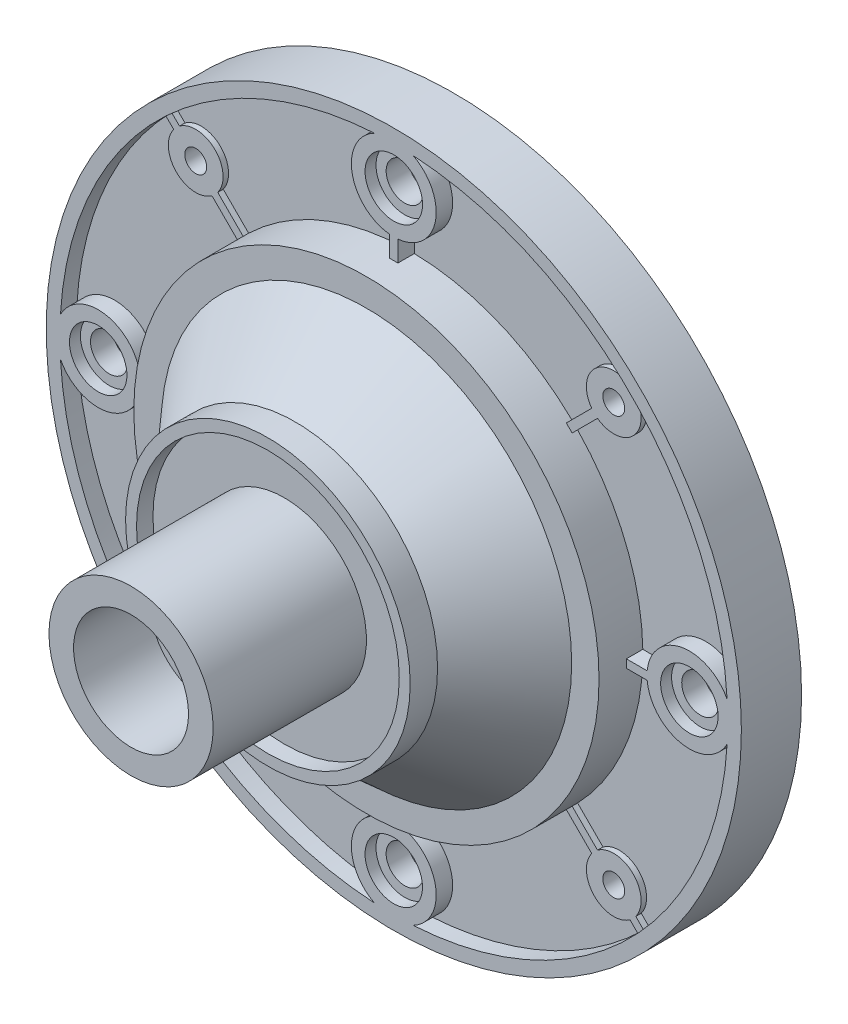
from build123d import *
from build123d.topology import SkipClean

# Parameters (mm, degrees)
SKETCH1_R           = 15
BOSS_EXTRUDE1_DEPTH = 30
SKETCH8_R           = 12
BOSS_EXTRUDE3_DEPTH = 20
SKETCH9_R           = 10.5
CUT_EXTRUDE3_DEPTH  = 14
SKETCH10_R          = 8.5
CUT_EXTRUDE4_DEPTH  = 42
SKETCH12_R          = 5.25
CUT_EXTRUDE5_DEPTH  = 2
SKETCH13_R          = 3.4
CUT_EXTRUDE6_DEPTH  = 16
CIRPATTERN1_COUNT   = 4
SKETCH15_R          = 5
CUT_EXTRUDE7_DEPTH  = 2
SKETCH16_R          = 2
CUT_EXTRUDE8_DEPTH  = 2
CIRPATTERN2_COUNT   = 4
CUT_EXTRUDE9_DEPTH  = 3
CUT_EXTRUDE10_DEPTH = 2
SKETCH19_R          = 2
CUT_EXTRUDE11_DEPTH = 36
SKETCH20_R          = 5.25
SKETCH20_R_2        = 3.4
BOSS_EXTRUDE4_DEPTH = 1
BOSS_EXTRUDE5_DEPTH = 12
BOSS_EXTRUDE6_REACH = 104.301
CIRPATTERN3_COUNT   = 8
BOSS_EXTRUDE9_START = -5
SKETCH25_W          = 1
SKETCH25_H          = 4.369199075
BOSS_EXTRUDE9_DEPTH = 3
CIRPATTERN4_COUNT   = 8


with BuildPart() as part:
    # Sketch1 → Boss-Extrude1 (new body)
    with BuildSketch(Plane.XY):
        Circle(SKETCH1_R)
    extrude(amount=BOSS_EXTRUDE1_DEPTH)

    # Sketch8 → Boss-Extrude3 (add)
    with BuildSketch(Plane(origin=(0, 0, 0), x_dir=(-1, 0, 0), z_dir=(0, 0, -1))):
        Circle(SKETCH8_R)
    extrude(amount=BOSS_EXTRUDE3_DEPTH)

    # Sketch9 → Cut-Extrude3 (cut)
    with BuildSketch(Plane.XY.offset(30)):
        Circle(SKETCH9_R)
    extrude(amount=-CUT_EXTRUDE3_DEPTH, mode=Mode.SUBTRACT)

    # Sketch10 → Cut-Extrude4 (cut)
    with BuildSketch(Plane.XY.offset(16)):
        Circle(SKETCH10_R)
    extrude(amount=-CUT_EXTRUDE4_DEPTH, mode=Mode.SUBTRACT)

    # Sketch11 → Revolve1 (revolve)
    with BuildSketch(Plane(origin=(0, 0, 0), x_dir=(0, 0, -1), z_dir=(1, 0, 0)), mode=Mode.PRIVATE) as revolve1_sk:
        Polygon((0, 12), (0, 23.329760776), (13.757661732, 35.5), (26, 35.5), (26, 37.5), (15, 37.5), (15, 40.5), (23, 40.5), (23, 61.5), (29, 61.5), (29, 63.5), (18, 63.5), (18, 42.5), (13, 42.5), (13, 37.5), (0, 26), (-5, 26), (-5, 24), (-2, 24), (-2, 15), align=None)
    revolve(revolve1_sk.sketch.rotate(Axis((0, 0, 37.815119145), (0, 0, -1)), 90), axis=Axis((0, 0, 37.815119145), (0, 0, -1)))

    # Sketch12 → Cut-Extrude5 (cut)
    with BuildSketch(Plane.XY.offset(-18)):
        with Locations((0, 54)):
            Circle(SKETCH12_R)
    cut_extrude5 = extrude(amount=-CUT_EXTRUDE5_DEPTH, mode=Mode.SUBTRACT)

    # Sketch13 → Cut-Extrude6 (cut)
    with BuildSketch(Plane.XY.offset(-20)):
        with Locations((0, 54)):
            Circle(SKETCH13_R)
    cut_extrude6 = extrude(amount=-CUT_EXTRUDE6_DEPTH, mode=Mode.SUBTRACT)

    # CirPattern1: Cut-Extrude5, Cut-Extrude6 ×4 about axis
    cirpattern1_axis = Axis((0, 0, 0), (0, 0, 1))
    add([cut_extrude5.rotate(cirpattern1_axis, i * 360 / CIRPATTERN1_COUNT) for i in range(1, CIRPATTERN1_COUNT)], mode=Mode.SUBTRACT)
    add([cut_extrude6.rotate(cirpattern1_axis, i * 360 / CIRPATTERN1_COUNT) for i in range(1, CIRPATTERN1_COUNT)], mode=Mode.SUBTRACT)

    # Sketch15 → Cut-Extrude7 (cut)
    with BuildSketch(Plane.XY.offset(-18)):
        with Locations((-38.183766184, 38.183766184)):
            Circle(SKETCH15_R)
    cut_extrude7 = extrude(amount=-CUT_EXTRUDE7_DEPTH, mode=Mode.SUBTRACT)

    # Sketch16 → Cut-Extrude8 (cut)
    with BuildSketch(Plane.XY.offset(-20)):
        with Locations((-38.183766184, 38.183766184)):
            Circle(SKETCH16_R)
    cut_extrude8 = extrude(amount=-CUT_EXTRUDE8_DEPTH, mode=Mode.SUBTRACT)

    # CirPattern2: Cut-Extrude7, Cut-Extrude8 ×4 about axis
    cirpattern2_axis = Axis((0, 0, 0), (0, 0, 1))
    add([cut_extrude7.rotate(cirpattern2_axis, i * 360 / CIRPATTERN2_COUNT) for i in range(1, CIRPATTERN2_COUNT)], mode=Mode.SUBTRACT)
    add([cut_extrude8.rotate(cirpattern2_axis, i * 360 / CIRPATTERN2_COUNT) for i in range(1, CIRPATTERN2_COUNT)], mode=Mode.SUBTRACT)

    # Sketch17 → Cut-Extrude9 (cut)
    with BuildSketch(Plane.XY.offset(-18)):
        with BuildLine():
            Line((-46.28637569, 0.75), (-42.493381838, 0.75))
            ThreePointArc((-42.493381838, 0.75), (-39.264880132, 16.264045876), (-30.577688539, 29.517028367))
            Line((-30.577688539, 29.517028367), (-35.218563406, 34.157903235))
            ThreePointArc((-35.218563406, 34.157903235), (-41.71930009, 34.648232278), (-42.209629133, 41.148968962))
            Line((-42.209629133, 41.148968962), (-43.660583389, 42.599923217))
            ThreePointArc((-43.660583389, 42.599923217), (-55.809022961, 24.624235139), (-60.897569444, 3.533558512))
            ThreePointArc((-60.897569444, 3.533558512), (-52.549642843, 7.613078491), (-46.28637569, 0.75))
        make_face()
        with BuildLine():
            Line((-43.660583389, -42.599923217), (-42.209629133, -41.148968962))
            ThreePointArc((-42.209629133, -41.148968962), (-41.71930009, -34.648232278), (-35.218563406, -34.157903235))
            Line((-35.218563406, -34.157903235), (-30.577688539, -29.517028367))
            ThreePointArc((-30.577688539, -29.517028367), (-39.264880132, -16.264045876), (-42.493381838, -0.75))
            Line((-42.493381838, -0.75), (-46.28637569, -0.75))
            ThreePointArc((-46.28637569, -0.75), (-52.549642843, -7.613078491), (-60.897569444, -3.533558512))
            ThreePointArc((-60.897569444, -3.533558512), (-55.809022961, -24.624235139), (-43.660583389, -42.599923217))
        make_face()
        with BuildLine():
            Line((-34.157903235, 35.218563406), (-29.517028367, 30.577688539))
            ThreePointArc((-29.517028367, 30.577688539), (-16.264045876, 39.264880132), (-0.75, 42.493381838))
            Line((-0.75, 42.493381838), (-0.75, 46.28637569))
            ThreePointArc((-0.75, 46.28637569), (-7.613078491, 52.549642843), (-3.533558512, 60.897569444))
            ThreePointArc((-3.533558512, 60.897569444), (-24.624235139, 55.809022961), (-42.599923217, 43.660583389))
            Line((-42.599923217, 43.660583389), (-41.148968962, 42.209629133))
            ThreePointArc((-41.148968962, 42.209629133), (-35.92832985, 42.64616542), (-33.183766184, 38.183766184))
            ThreePointArc((-33.183766184, 38.183766184), (-33.433539098, 36.62320775), (-34.157903235, 35.218563406))
        make_face()
        with BuildLine():
            Line((0.75, 46.28637569), (0.75, 42.493381838))
            ThreePointArc((0.75, 42.493381838), (16.264045876, 39.264880132), (29.517028367, 30.577688539))
            Line((29.517028367, 30.577688539), (34.157903235, 35.218563406))
            ThreePointArc((34.157903235, 35.218563406), (34.648232278, 41.71930009), (41.148968962, 42.209629133))
            Line((41.148968962, 42.209629133), (42.599923217, 43.660583389))
            ThreePointArc((42.599923217, 43.660583389), (24.624235139, 55.809022961), (3.533558512, 60.897569444))
            ThreePointArc((3.533558512, 60.897569444), (7.613078491, 52.549642843), (0.75, 46.28637569))
        make_face()
        with BuildLine():
            ThreePointArc((30.577688539, 29.517028367), (39.264880132, 16.264045876), (42.493381838, 0.75))
            Line((42.493381838, 0.75), (46.28637569, 0.75))
            ThreePointArc((46.28637569, 0.75), (52.549642843, 7.613078491), (60.897569444, 3.533558512))
            ThreePointArc((60.897569444, 3.533558512), (55.809022961, 24.624235139), (43.660583389, 42.599923217))
            Line((43.660583389, 42.599923217), (42.209629133, 41.148968962))
            ThreePointArc((42.209629133, 41.148968962), (42.933993271, 39.744324618), (43.183766184, 38.183766184))
            ThreePointArc((43.183766184, 38.183766184), (40.439202518, 33.721366948), (35.218563406, 34.157903235))
            Line((35.218563406, 34.157903235), (30.577688539, 29.517028367))
        make_face()
        with BuildLine():
            ThreePointArc((43.183766184, -38.183766184), (42.933993271, -39.744324618), (42.209629133, -41.148968962))
            Line((42.209629133, -41.148968962), (43.660583389, -42.599923217))
            ThreePointArc((43.660583389, -42.599923217), (55.809022961, -24.624235139), (60.897569444, -3.533558512))
            ThreePointArc((60.897569444, -3.533558512), (52.549642843, -7.613078491), (46.28637569, -0.75))
            Line((46.28637569, -0.75), (42.493381838, -0.75))
            ThreePointArc((42.493381838, -0.75), (39.264880132, -16.264045876), (30.577688539, -29.517028367))
            Line((30.577688539, -29.517028367), (35.218563406, -34.157903235))
            ThreePointArc((35.218563406, -34.157903235), (40.439202518, -33.721366948), (43.183766184, -38.183766184))
        make_face()
        with BuildLine():
            ThreePointArc((0.75, -46.28637569), (7.613078491, -52.549642843), (3.533558512, -60.897569444))
            ThreePointArc((3.533558512, -60.897569444), (24.624235139, -55.809022961), (42.599923217, -43.660583389))
            Line((42.599923217, -43.660583389), (41.148968962, -42.209629133))
            ThreePointArc((41.148968962, -42.209629133), (34.648232278, -41.71930009), (34.157903235, -35.218563406))
            Line((34.157903235, -35.218563406), (29.517028367, -30.577688539))
            ThreePointArc((29.517028367, -30.577688539), (16.264045876, -39.264880132), (0.75, -42.493381838))
            Line((0.75, -42.493381838), (0.75, -46.28637569))
        make_face()
        with BuildLine():
            ThreePointArc((-33.183766184, -38.183766184), (-35.92832985, -42.64616542), (-41.148968962, -42.209629133))
            Line((-41.148968962, -42.209629133), (-42.599923217, -43.660583389))
            ThreePointArc((-42.599923217, -43.660583389), (-24.624235139, -55.809022961), (-3.533558512, -60.897569444))
            ThreePointArc((-3.533558512, -60.897569444), (-7.613078491, -52.549642843), (-0.75, -46.28637569))
            Line((-0.75, -46.28637569), (-0.75, -42.493381838))
            ThreePointArc((-0.75, -42.493381838), (-16.264045876, -39.264880132), (-29.517028367, -30.577688539))
            Line((-29.517028367, -30.577688539), (-34.157903235, -35.218563406))
            ThreePointArc((-34.157903235, -35.218563406), (-33.433539098, -36.62320775), (-33.183766184, -38.183766184))
        make_face()
    extrude(amount=-CUT_EXTRUDE9_DEPTH, mode=Mode.SUBTRACT)

    # Sketch18 → Cut-Extrude10 (cut)
    with BuildSketch(Plane.XY.offset(-18)):
        with BuildLine():
            Line((-43.660583389, 42.599923217), (-42.209629133, 41.148968962))
            ThreePointArc((-42.209629133, 41.148968962), (-41.71930009, 41.71930009), (-41.148968962, 42.209629133))
            Line((-41.148968962, 42.209629133), (-42.599923217, 43.660583389))
            ThreePointArc((-42.599923217, 43.660583389), (-43.133513652, 43.133513652), (-43.660583389, 42.599923217))
        make_face()
        with BuildLine():
            ThreePointArc((-30.577688539, 29.517028367), (-30.0520382, 30.0520382), (-29.517028367, 30.577688539))
            Line((-29.517028367, 30.577688539), (-34.157903235, 35.218563406))
            ThreePointArc((-34.157903235, 35.218563406), (-34.648232278, 34.648232278), (-35.218563406, 34.157903235))
            Line((-35.218563406, 34.157903235), (-30.577688539, 29.517028367))
        make_face()
        with BuildLine():
            Line((42.599923217, 43.660583389), (41.148968962, 42.209629133))
            ThreePointArc((41.148968962, 42.209629134), (41.71930009, 41.71930009), (42.209629134, 41.148968962))
            Line((42.209629133, 41.148968962), (43.660583389, 42.599923217))
            ThreePointArc((43.660583389, 42.599923217), (43.133513652, 43.133513652), (42.599923217, 43.660583389))
        make_face()
        with BuildLine():
            Line((34.157903235, 35.218563406), (29.517028367, 30.577688539))
            ThreePointArc((29.517028367, 30.577688539), (30.0520382, 30.0520382), (30.577688539, 29.517028367))
            Line((30.577688539, 29.517028367), (35.218563406, 34.157903235))
            ThreePointArc((35.218563406, 34.157903235), (34.648232278, 34.648232278), (34.157903235, 35.218563406))
        make_face()
        with BuildLine():
            Line((35.218563406, -34.157903235), (30.577688539, -29.517028367))
            ThreePointArc((30.577688539, -29.517028367), (30.0520382, -30.0520382), (29.517028367, -30.577688539))
            Line((29.517028367, -30.577688539), (34.157903235, -35.218563406))
            ThreePointArc((34.157903235, -35.218563406), (34.648232278, -34.648232278), (35.218563406, -34.157903235))
        make_face()
        with BuildLine():
            ThreePointArc((42.209629134, -41.148968962), (41.71930009, -41.71930009), (41.148968962, -42.209629133))
            Line((41.148968962, -42.209629133), (42.599923217, -43.660583389))
            ThreePointArc((42.599923217, -43.660583389), (43.133513652, -43.133513652), (43.660583389, -42.599923217))
            Line((43.660583389, -42.599923217), (42.209629133, -41.148968962))
        make_face()
        with BuildLine():
            ThreePointArc((-41.148968962, -42.209629133), (-41.71930009, -41.71930009), (-42.209629133, -41.148968962))
            Line((-42.209629133, -41.148968962), (-43.660583389, -42.599923217))
            ThreePointArc((-43.660583389, -42.599923217), (-43.133513652, -43.133513652), (-42.599923217, -43.660583389))
            Line((-42.599923217, -43.660583389), (-41.148968962, -42.209629133))
        make_face()
        with BuildLine():
            ThreePointArc((-29.517028367, -30.577688539), (-30.0520382, -30.0520382), (-30.577688539, -29.517028367))
            Line((-30.577688539, -29.517028367), (-35.218563406, -34.157903235))
            ThreePointArc((-35.218563406, -34.157903235), (-34.648232278, -34.648232278), (-34.157903235, -35.218563406))
            Line((-34.157903235, -35.218563406), (-29.517028367, -30.577688539))
        make_face()
    extrude(amount=-CUT_EXTRUDE10_DEPTH, mode=Mode.SUBTRACT)

    # Sketch19 → Cut-Extrude11 (cut)
    with BuildSketch(Plane.XY.offset(-20)):
        with Locations((-38.183766184, 38.183766184)):
            Circle(SKETCH19_R)
        with Locations((-38.183766184, -38.183766184)):
            Circle(SKETCH19_R)
        with Locations((38.183766184, -38.183766184)):
            Circle(SKETCH19_R)
        with Locations((38.183766184, 38.183766184)):
            Circle(SKETCH19_R)
    extrude(amount=-CUT_EXTRUDE11_DEPTH, mode=Mode.SUBTRACT)

    # Sketch20 → Boss-Extrude4 (add)
    # profile 1 of 4: a face of its own
    with BuildSketch(Plane(origin=(0, 0, -23), x_dir=(-1, 0, 0), z_dir=(0, 0, -1))):
        with Locations(Location((0, 54, 0), (0, 0, 180))):
            Circle(SKETCH20_R)
        with Locations(Location((0, 54, 0), (0, 0, 180))):
            Circle(SKETCH20_R_2, mode=Mode.SUBTRACT)
    # profile 2 of 4: a face of its own
    with BuildSketch(Plane(origin=(0, 0, -23), x_dir=(-1, 0, 0), z_dir=(0, 0, -1))):
        with Locations(Location((-54, 0, 0), (0, 0, 270))):
            Circle(SKETCH20_R)
        with Locations(Location((-54, 0, 0), (0, 0, 270))):
            Circle(SKETCH20_R_2, mode=Mode.SUBTRACT)
    # profile 3 of 4: a face of its own
    with BuildSketch(Plane(origin=(0, 0, -23), x_dir=(-1, 0, 0), z_dir=(0, 0, -1))):
        with Locations((0, -54)):
            Circle(SKETCH20_R)
        with Locations((0, -54)):
            Circle(SKETCH20_R_2, mode=Mode.SUBTRACT)
    # profile 4 of 4: a face of its own
    with BuildSketch(Plane(origin=(0, 0, -23), x_dir=(-1, 0, 0), z_dir=(0, 0, -1))):
        with Locations(Location((54, 0, 0), (0, 0, 90))):
            Circle(SKETCH20_R)
        with Locations(Location((54, 0, 0), (0, 0, 90))):
            Circle(SKETCH20_R_2, mode=Mode.SUBTRACT)
    extrude(amount=BOSS_EXTRUDE4_DEPTH)

    # Sketch21 → Boss-Extrude5 (add)
    with SkipClean():  # the faces are left unmerged after this step: merging them gives an invalid solid
        with BuildSketch(Plane(origin=(0, 0, -26), x_dir=(-1, 0, 0), z_dir=(0, 0, -1))):
            with BuildLine():
                ThreePointArc((-28.387596195, 21.316528383), (-25.102290732, 25.102290732), (-21.316528383, 28.387596195))
                Line((-21.316528383, 28.387596195), (-22.744211146, 29.815278958))
                ThreePointArc((-22.744211146, 29.815278958), (-26.516504294, 26.516504294), (-29.815278958, 22.744211146))
                Line((-29.815278958, 22.744211146), (-28.387596195, 21.316528383))
            make_face()
            with BuildLine():
                Line((26.516504294, 26.516504294), (25.102290732, 25.102290732))
                ThreePointArc((25.102290732, 25.102290732), (26.811844398, 23.267466557), (28.387596195, 21.316528383))
                Line((28.387596195, 21.316528383), (29.815278958, 22.744211146))
                ThreePointArc((29.815278958, 22.744211146), (28.228974477, 24.685522073), (26.516504294, 26.516504294))
            make_face()
            with BuildLine():
                ThreePointArc((21.316528383, 28.387596195), (23.267466557, 26.811844398), (25.102290732, 25.102290732))
                Line((25.102290732, 25.102290732), (26.516504294, 26.516504294))
                ThreePointArc((26.516504294, 26.516504294), (24.685522073, 28.228974477), (22.744211146, 29.815278958))
                Line((22.744211146, 29.815278958), (21.316528383, 28.387596195))
            make_face()
            with BuildLine():
                Line((29.815278958, -22.744211146), (28.387596195, -21.316528383))
                ThreePointArc((28.387596195, -21.316528383), (25.102290732, -25.102290732), (21.316528383, -28.387596195))
                Line((21.316528383, -28.387596195), (22.744211146, -29.815278958))
                ThreePointArc((22.744211146, -29.815278958), (26.516504294, -26.516504294), (29.815278958, -22.744211146))
            make_face()
            with BuildLine():
                ThreePointArc((-28.387596195, -21.316528383), (-25.102290732, -25.102290732), (-21.316528383, -28.387596195))
                Line((-21.316528383, -28.387596195), (-22.744211146, -29.815278958))
                ThreePointArc((-22.744211146, -29.815278958), (-26.516504294, -26.516504294), (-29.815278958, -22.744211146))
                Line((-29.815278958, -22.744211146), (-28.387596195, -21.316528383))
            make_face()
        extrude(amount=BOSS_EXTRUDE5_DEPTH)

    # Boss-Extrude6: up to this face of the body (flat: up to its plane)
    boss_extrude6_end = Plane(part.part.faces().sort_by_distance((12.659865282, 0, 0))[0])
    # Sketch22 → Boss-Extrude6 (add, up to the picked face)
    with BuildSketch(Plane(origin=(0, 0, -19), x_dir=(-1, 0, 0), z_dir=(0, 0, -1)), mode=Mode.PRIVATE) as boss_extrude6_sk1:
        with BuildLine():
            Line((-0.5, 35.496478699), (-0.5, 11.989578808))
            ThreePointArc((-0.5, 11.989578808), (0, 12), (0.5, 11.989578808))
            Line((0.5, 11.989578808), (0.5, 35.496478699))
            ThreePointArc((0.5, 35.496478699), (0, 35.5), (-0.5, 35.496478699))
        make_face()
    boss_extrude6_tool1 = split(extrude(boss_extrude6_sk1.sketch, amount=-BOSS_EXTRUDE6_REACH, mode=Mode.PRIVATE), bisect_by=boss_extrude6_end, keep=Keep.BOTH, mode=Mode.PRIVATE)
    boss_extrude6 = boss_extrude6_tool1.solids().sort_by(Axis((0, 23.747676, -19), (0, 0, 1)))[0]
    add(boss_extrude6)

    # Sketch23 → Cut-Revolve1 (revolve, cut)
    with SkipClean():  # the faces are left unmerged after this step: merging them gives an invalid solid
        with BuildSketch(Plane(origin=(0, 0, 0), x_dir=(0, 0, -1), z_dir=(1, 0, 0)), mode=Mode.PRIVATE) as cut_revolve1_sk:
            with BuildLine():
                Line((13, 37.5), (0, 25.995191863))
                Line((0, 25.995191863), (0, 39.76109473))
                Line((0, 39.76109473), (12.775523961, 37.699520548))
                ThreePointArc((12.775523961, 37.699520548), (12.832991792, 37.538139579), (13, 37.5))
            make_face()
        cut_revolve1 = revolve(cut_revolve1_sk.sketch.rotate(Axis((0, 0, 38.61502355), (0, 0, -1)), 2.388015463), axis=Axis((0, 0, 38.61502355), (0, 0, -1)), mode=Mode.SUBTRACT)

    # CirPattern3: Boss-Extrude6, Cut-Revolve1 ×8 about axis
    with SkipClean():  # the faces are left unmerged after this step: merging them gives an invalid solid
        cirpattern3_axis = Axis((0, 0, 0), (0, 0, 1))
        add([boss_extrude6.rotate(cirpattern3_axis, i * 360 / CIRPATTERN3_COUNT) for i in range(1, CIRPATTERN3_COUNT)])
        add([cut_revolve1.rotate(cirpattern3_axis, i * 360 / CIRPATTERN3_COUNT) for i in range(1, CIRPATTERN3_COUNT)], mode=Mode.SUBTRACT)

    # Sketch25 → Boss-Extrude9 (add)
    with SkipClean():  # the faces are left unmerged after this step: merging them gives an invalid solid
        with BuildSketch(Plane(origin=(0, 0, -23), x_dir=(-1, 0, 0), z_dir=(0, 0, -1)).offset(BOSS_EXTRUDE9_START)):
            with Locations((0, 38.728547351)):
                Rectangle(SKETCH25_W, SKETCH25_H)
        boss_extrude9 = extrude(amount=-BOSS_EXTRUDE9_DEPTH)

    # CirPattern4: Boss-Extrude9 ×8 about axis
    with SkipClean():  # the faces are left unmerged after this step: merging them gives an invalid solid
        cirpattern4_axis = Axis((0, 0, 0), (0, 0, 1))
        for i in range(1, CIRPATTERN4_COUNT):
            add(boss_extrude9.rotate(cirpattern4_axis, i * 360 / CIRPATTERN4_COUNT))


solid = part.part
